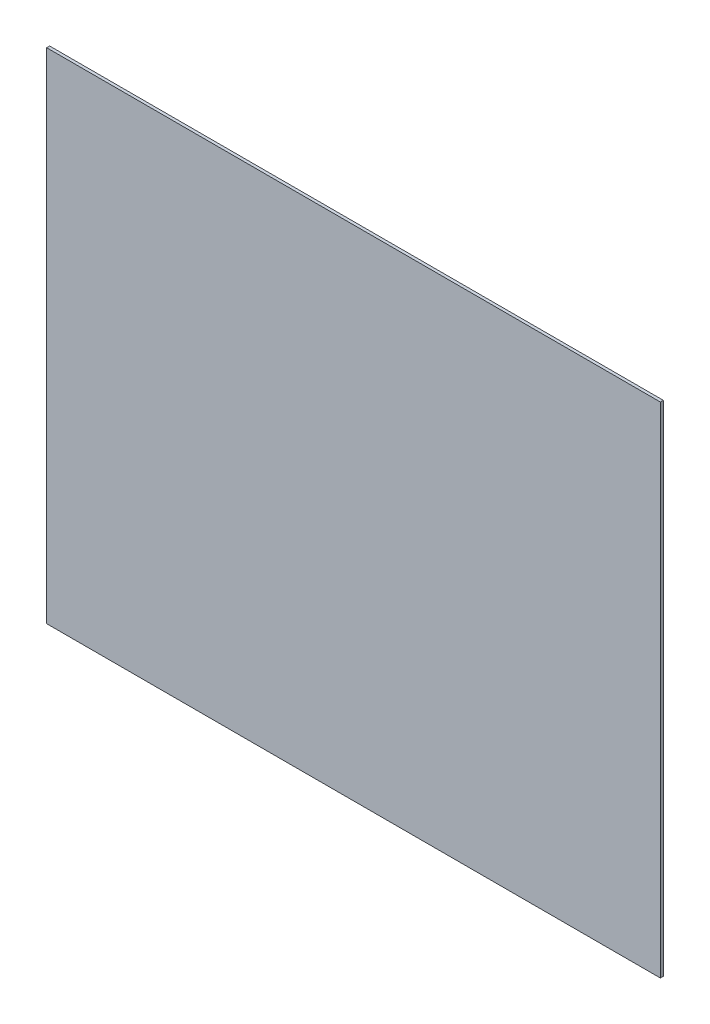
from build123d import *

# Parameters (mm, degrees)
SKETCH_1_W      = 1037
SKETCH_1_H      = 843
EXTRUDE_1_DEPTH = 5


with BuildPart() as part:
    # 草图1 → 凸台-拉伸1 (new body)
    with BuildSketch(Plane.XY):
        Rectangle(SKETCH_1_W, SKETCH_1_H)
    extrude(amount=EXTRUDE_1_DEPTH)


solid = part.part
